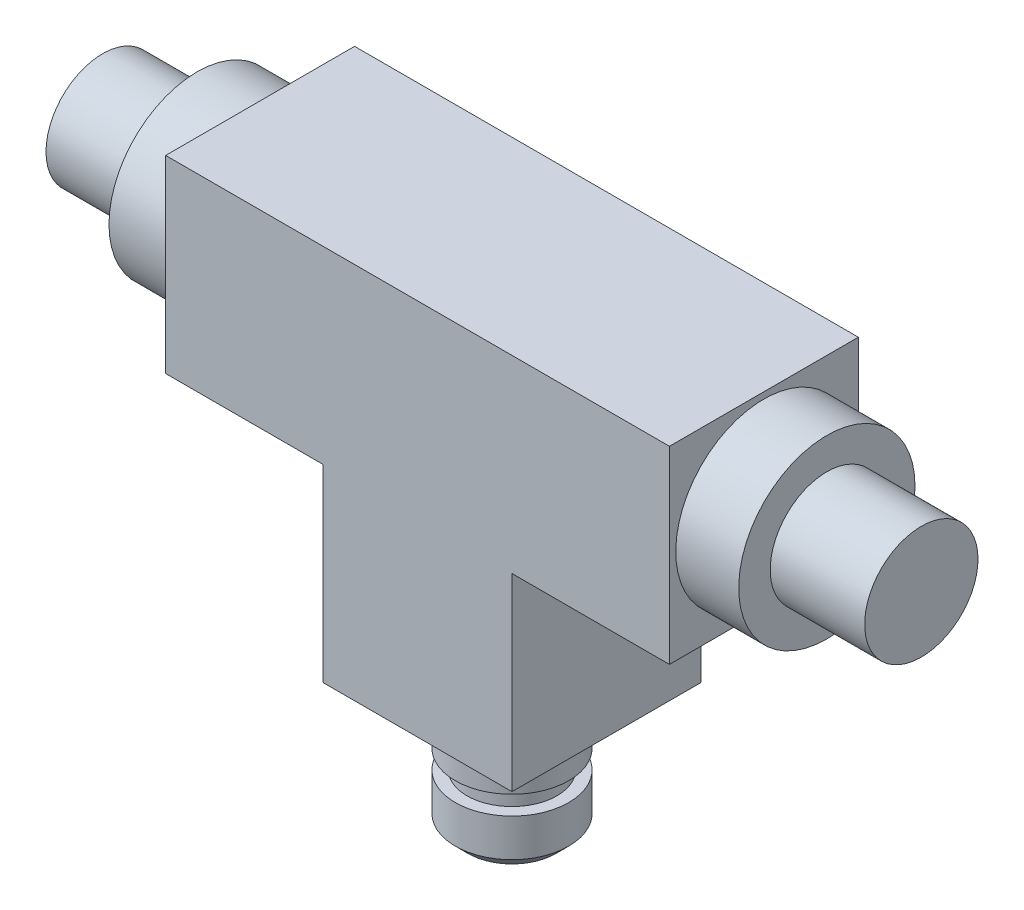
from build123d import *

# Parameters (mm, degrees)
BOSS_EXTRUDE1_DEPTH = 30
SKETCH2_R           = 14
BOSS_EXTRUDE2_DEPTH = 10
SKETCH3_R           = 9
BOSS_EXTRUDE3_DEPTH = 15
BOSS_EXTRUDE4_START = 10
SKETCH4_R           = 14
BOSS_EXTRUDE4_DEPTH = 10
BOSS_EXTRUDE5_START = 15
SKETCH5_R           = 9
BOSS_EXTRUDE5_DEPTH = 15
SKETCH6_R           = 9
BOSS_EXTRUDE6_DEPTH = 20
CUT_EXTRUDE1_START  = -8
SKETCH7_R           = 10.265478639
SKETCH7_R_2         = 7.147971295
CUT_EXTRUDE1_DEPTH  = 3
CHAMFER1_SIZE       = 2
SKETCH8_R           = 2.5
CUT_EXTRUDE2_DEPTH  = 6


with BuildPart() as part:
    # Sketch1 → Boss-Extrude1 (new body)
    with BuildSketch(Plane.XY):
        Polygon((0, 0), (0, 30), (-25, 30), (-25, 60), (55, 60), (55, 30), (30, 30), (30, 0), align=None)
    extrude(amount=BOSS_EXTRUDE1_DEPTH)

    # Sketch2 → Boss-Extrude2 (add)
    with BuildSketch(Plane(origin=(55, 0, 0), x_dir=(0, 0, -1), z_dir=(1, 0, 0))):
        with Locations(Location((-15, 45, 0), (0, 0, 270))):
            Circle(SKETCH2_R)
    extrude(amount=BOSS_EXTRUDE2_DEPTH)

    # Sketch3 → Boss-Extrude3 (add)
    with BuildSketch(Plane(origin=(65, 0, 0), x_dir=(0, 0, -1), z_dir=(1, 0, 0))):
        with Locations((-15, 45)):
            Circle(SKETCH3_R)
    extrude(amount=BOSS_EXTRUDE3_DEPTH)

    # Sketch4 → Boss-Extrude4 (add)
    with BuildSketch(Plane.ZY.offset(25).offset(BOSS_EXTRUDE4_START)):
        with Locations(Location((15, 45, 0), (0, 0, 270))):
            Circle(SKETCH4_R)
    extrude(amount=-BOSS_EXTRUDE4_DEPTH)

    # Sketch5 → Boss-Extrude5 (add)
    with BuildSketch(Plane.ZY.offset(35).offset(BOSS_EXTRUDE5_START)):
        with Locations(Location((15, 45, 0), (0, 0, 180))):
            Circle(SKETCH5_R)
    extrude(amount=-BOSS_EXTRUDE5_DEPTH)

    # Sketch6 → Boss-Extrude6 (add)
    with BuildSketch(Plane(origin=(0, 0, 0), x_dir=(-1, 0, 0), z_dir=(0, -1, 0))):
        with Locations((-15, -15)):
            Circle(SKETCH6_R)
    extrude(amount=BOSS_EXTRUDE6_DEPTH)

    # Sketch7 → Cut-Extrude1 (cut)
    with BuildSketch(Plane(origin=(0, -20, 0), x_dir=(-1, 0, 0), z_dir=(0, -1, 0)).offset(CUT_EXTRUDE1_START)):
        with Locations((-15, -15)):
            Circle(SKETCH7_R)
        with Locations(Location((-15, -15, 0), (0, 0, 180))):
            Circle(SKETCH7_R_2, mode=Mode.SUBTRACT)
    extrude(amount=-CUT_EXTRUDE1_DEPTH, mode=Mode.SUBTRACT)

    # Chamfer1
    chamfer1_edges = [part.edges().sort_by_distance(p)[0] for p in [
        (24, -20, 15),
    ]]
    chamfer(chamfer1_edges, length=CHAMFER1_SIZE)

    # Sketch8 → Cut-Extrude2 (cut)
    with BuildSketch(Plane(origin=(0, 0, 0), x_dir=(-1, 0, 0), z_dir=(0, 0, -1))):
        with Locations((-50, 45)):
            Circle(SKETCH8_R)
        with Locations((20, 45)):
            Circle(SKETCH8_R)
    extrude(amount=-CUT_EXTRUDE2_DEPTH, mode=Mode.SUBTRACT)


solid = part.part
